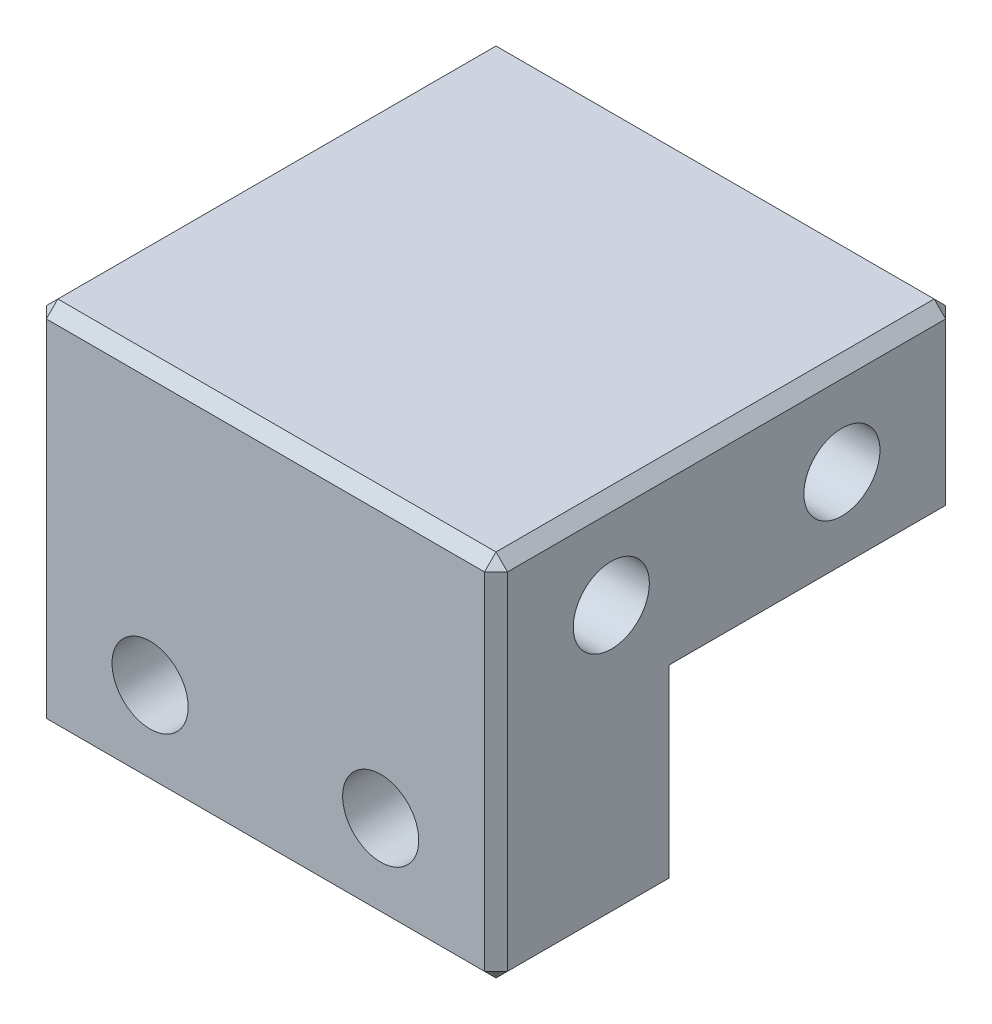
SolidWorks part; units mm, degrees
material "Al6061"
ref_plane "Front" through (0, 0, 0) normal (0, 0, 1) x (1, 0, 0)
ref_plane "Top" through (0, 0, 0) normal (0, 1, 0) x (1, 0, 0)
ref_plane "Right" through (0, 0, 0) normal (1, 0, 0) x (0, 0, -1)
sketch "草图1" plane through (0, 0, 0) normal (0, 1, 0) x (1, 0, 0)
  line L1 (-10, 10) -> (10, 10)
  line L2 (-10, 10) -> (-10, -10)
  line L3 (-10, -10) -> (10, -10)
  line L4 (10, 10) -> (10, -10)
  line L5 (-10, 10) -> (10, -10) construction
  line L6 (-10, -10) -> (10, 10) construction
  point P0 (0, 0)
  dimension "D1" = 20
  dimension "D2" = 20
extrude "凸台-拉伸1" add sketch "草图1" along normal blind 8
hole_wizard "M4 螺纹孔1" positions "草图3" profile "草图2" tap size "M4" standard "Gb"
sketch "草图3" plane through (10, 0, 0) normal (1, 0, 0) x (0, 0, -1)
  line L1 (10, 4) -> (5, 4) construction
  line L3 (10, 8) -> (10, 0) construction
  point P0 (5, 4)
  point P2 (-5, 4)
  dimension "D1" = 5
  dimension "D2" = 10
sketch "草图2" plane through (10, 4, -5) normal (0, 1, 0) x (0, 0, -1)
  line L0 (0, 0) -> (0, 15.0914)
  line L1 (0, 15.0914) -> (1.65, 14.1)
  line L2 (1.65, 14.1) -> (1.65, 0)
  line L5 (1.65, 0) -> (0, 0)
  line L10 (0, 15.0914) -> (-1.65, 14.1) construction
  line L11 (0, -6.35) -> (0, 107.95) construction
  dimension "螺纹孔钻头直径" = 3.3
  dimension "螺纹孔钻头深度" = 14.1
  dimension "导头角度" = 118
cosmetic thread "孔螺蚊线1" parameters "D1"=12, "D2"=4
cosmetic thread "孔螺蚊线2" parameters "D1"=12, "D2"=4
sketch "草图6" plane through (0, 0, 10) normal (0, 0, 1) x (1, 0, 0)
  line L0 (10, 8) -> (10, 0) construction
  line L1 (-10, 0) -> (10, 0)
  line L2 (-10, 0) -> (-10, -8)
  line L3 (-10, -8) -> (10, -8)
  line L4 (10, 0) -> (10, -8)
  dimension "D1" = 8
extrude "凸台-拉伸2" add sketch "草图6" against normal blind 8
hole_wizard "M4 螺纹孔3" positions "草图8" profile "草图7" tap size "M4" standard "Gb"
sketch "草图8" plane through (0, 0, 10) normal (0, 0, 1) x (1, 0, 0)
  line L0 (-10, 8) -> (10, 8) construction
  line L1 (10, 8) -> (10, -8) construction
  point P0 (-5, -4)
  point P2 (5, -4)
  dimension "D1" = 12
  dimension "D2" = 5
  dimension "D3" = 10
sketch "草图7" plane through (-5, -4, 10) normal (1, 0, 0) x (0, -1, 0)
  line L0 (0, 0) -> (0, 15.0914)
  line L1 (0, 15.0914) -> (1.65, 14.1)
  line L2 (1.65, 14.1) -> (1.65, 0)
  line L5 (1.65, 0) -> (0, 0)
  line L10 (0, 15.0914) -> (-1.65, 14.1) construction
  line L11 (0, -6.35) -> (0, 107.95) construction
  dimension "螺纹孔钻头直径" = 3.3
  dimension "螺纹孔钻头深度" = 14.1
  dimension "导头角度" = 118
cosmetic thread "孔螺蚊线5" parameters "D1"=10, "D2"=4
cosmetic thread "孔螺蚊线6" parameters "D1"=10, "D2"=4
chamfer "倒角2" distance 0.5 angle 45 17 edges at (-10, 8, 0) (-10, 0, 10) (10, 4, -10) (0, 8, -10) (-10, 4, -10) (0, 0, -10) (10, -8, 6) (0, -8, 2) (-10, -8, 6) (0, -8, 10) (10, 8, 0) (0, 8, 10) (10, 0, 10)
